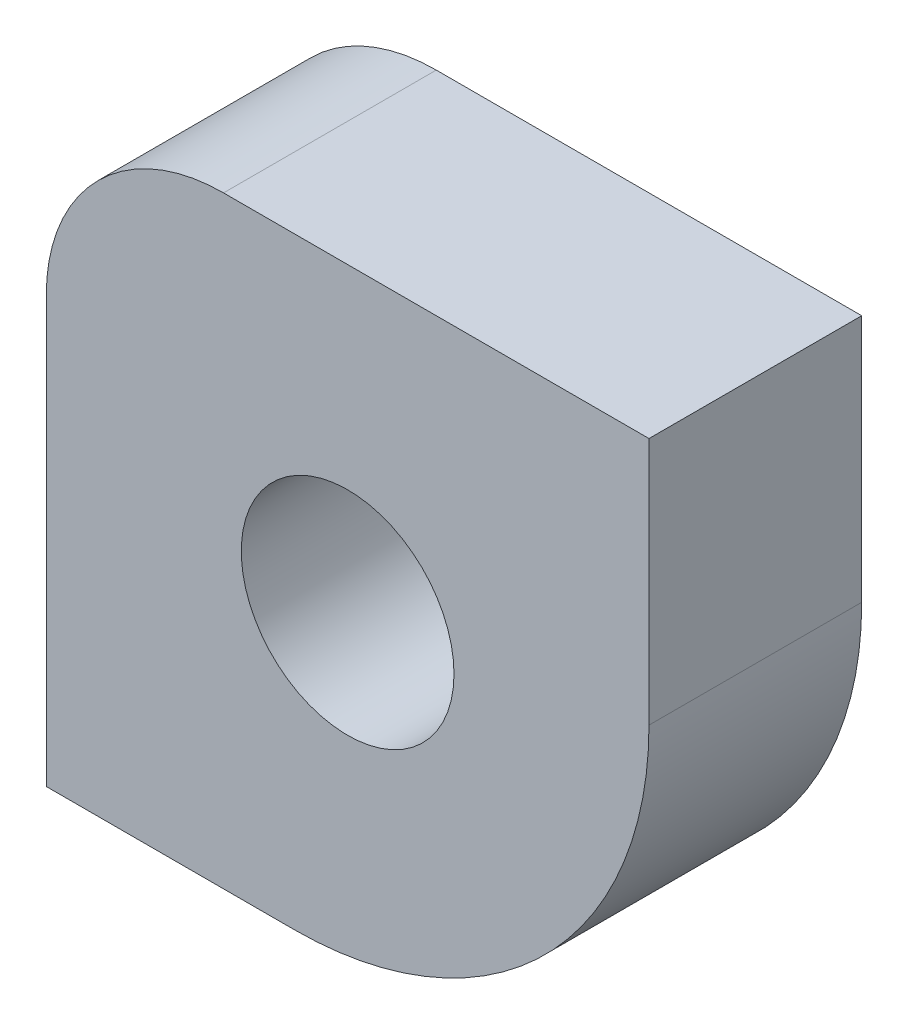
SolidWorks part; units mm, degrees
material "Plain Carbon Steel"
ref_plane "Front Plane" through (0, 0, 0) normal (0, 0, 1) x (1, 0, 0)
ref_plane "Top Plane" through (0, 0, 0) normal (0, 1, 0) x (1, 0, 0)
ref_plane "Right Plane" through (0, 0, 0) normal (1, 0, 0) x (0, 0, -1)
sketch "Sketch1" plane through (0, 0, 0) normal (0, 0, 1) x (1, 0, 0)
  line L1 (0, 0) -> (17, 0)
  line L2 (0, 0) -> (0, -17)
  line L3 (0, -17) -> (17, -17)
  line L4 (17, 0) -> (17, -17)
  dimension "D1" = 17
  dimension "D2" = 17
extrude "Boss-Extrude1" add sketch "Sketch1" along normal blind 6
fillet "Fillet1" radius 10 1 edges at (17, -17, 3)
fillet "Fillet2" radius 5 1 edges at (0, 0, 3)
sketch "Sketch2" plane through (0, 0, 6) normal (0, 0, 1) x (1, 0, 0)
  line L0 (0, -5) -> (0, -17) construction
  line L1 (17, 0) -> (5, 0) construction
  circle A0 centre (8.5, -8.5) radius 3
  dimension "D3" = 6
  dimension "D1" = 8.5
  dimension "D2" = 8.5
extrude "Cut-Extrude1" cut sketch "Sketch2" against normal blind 6
